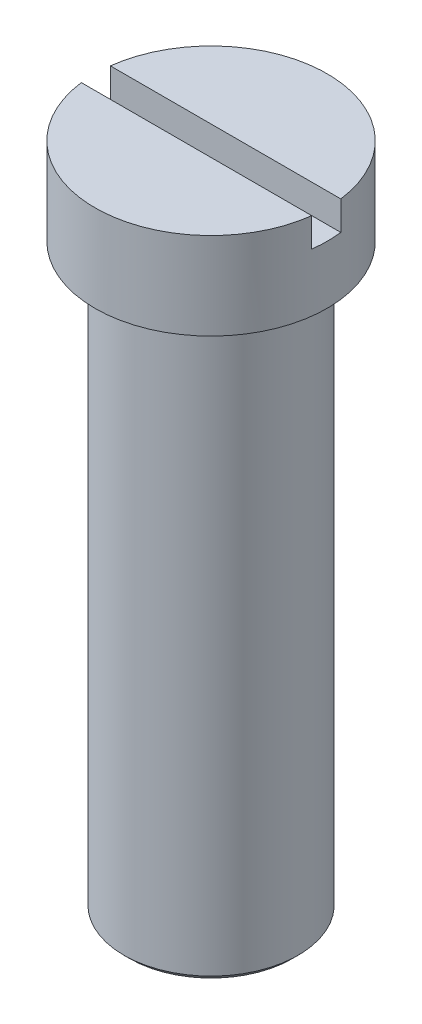
SolidWorks part; units mm, degrees
ref_plane "前视基准面" through (0, 0, 0) normal (0, 0, 1) x (1, 0, 0)
ref_plane "上视基准面" through (0, 0, 0) normal (0, 1, 0) x (1, 0, 0)
ref_plane "右视基准面" through (0, 0, 0) normal (1, 0, 0) x (0, 0, -1)
other "Configuration Table"
sketch "草图1" plane through (0, 0, 0) normal (0, 1, 0) x (1, 0, 0)
  circle A0 centre (0, 0) radius 15
  dimension "D1" = 30
extrude "凸台-拉伸1" add sketch "草图1" along normal mid plane 100 contours A0
sketch "草图2" plane through (0, 50, 0) normal (0, 1, 0) x (1, 0, 0)
  circle A0 centre (0, 0) radius 20
  dimension "D1" = 40
extrude "凸台-拉伸2" add sketch "草图2" along normal blind 15 contours A0
sketch "草图3" plane through (0, 65, 0) normal (0, 1, 0) x (1, 0, 0)
  line L1 (-30.0923, -2.5) -> (30.0923, -2.5)
  line L2 (-30.0923, -2.5) -> (-30.0923, 2.5)
  line L3 (-30.0923, 2.5) -> (30.0923, 2.5)
  line L4 (30.0923, -2.5) -> (30.0923, 2.5)
  line L5 (-30.0923, -2.5) -> (30.0923, 2.5) construction
  line L6 (-30.0923, 2.5) -> (30.0923, -2.5) construction
  point P0 (0, 0)
  dimension "D1" = 5
extrude "切除-拉伸1" cut sketch "草图3" against normal blind 5 contours L1 L4 L3 L2
chamfer "倒角1" distance 1 angle 45 1 edges at (0, -50, 15)
